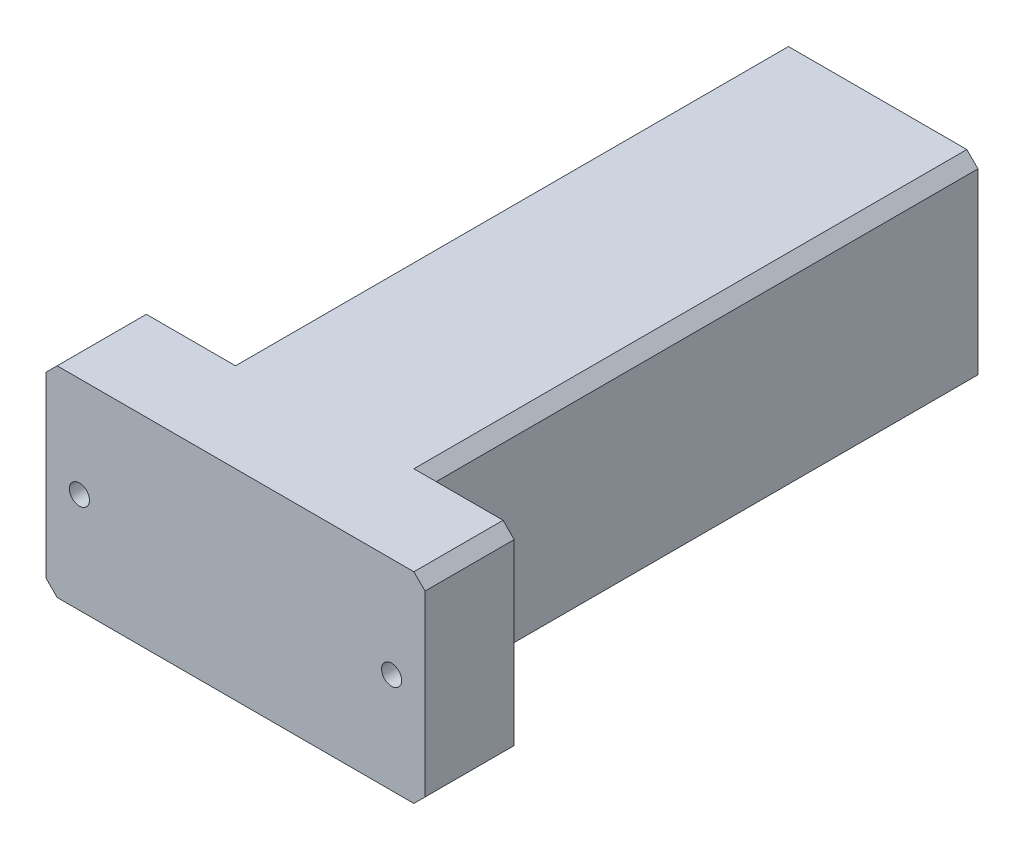
from build123d import *

# Parameters (mm, degrees)
SKETCH1_W            = 90
SKETCH1_H            = 90
BOSS_EXTRUDE1_DEPTH  = 288
SKETCH2_W            = 170
SKETCH2_H            = 90
BOSS_EXTRUDE2_DEPTH  = 40
CHAMFER1_SIZE        = 5
M8_CLEARANCE_HOLE1_D = 9


with BuildPart() as part:
    # Sketch1 → Boss-Extrude1 (new body)
    with BuildSketch(Plane.XY):
        Rectangle(SKETCH1_W, SKETCH1_H)
    extrude(amount=BOSS_EXTRUDE1_DEPTH)

    # Sketch2 → Boss-Extrude2 (add)
    with BuildSketch(Plane.XY.offset(288)):
        Rectangle(SKETCH2_W, SKETCH2_H)
    extrude(amount=-BOSS_EXTRUDE2_DEPTH)

    # Chamfer1
    chamfer1_edges = [part.edges().sort_by_distance(p)[0] for p in [
        (45, -45, 124),
        (-45, -45, 124),
        (-45, 45, 124),
        (45, 45, 124),
        (-85, 45, 268),
        (85, -45, 268),
        (-85, -45, 268),
        (85, 45, 268),
    ]]
    chamfer(chamfer1_edges, length=CHAMFER1_SIZE)

    # M8 Clearance Hole1 (through all)
    with Locations(Plane(origin=(0, 0, 248), x_dir=(-1, 0, 0), z_dir=(0, 0, -1))):
        with Locations((-70, 0), (70, 0)):
            Hole(M8_CLEARANCE_HOLE1_D / 2)


solid = part.part
